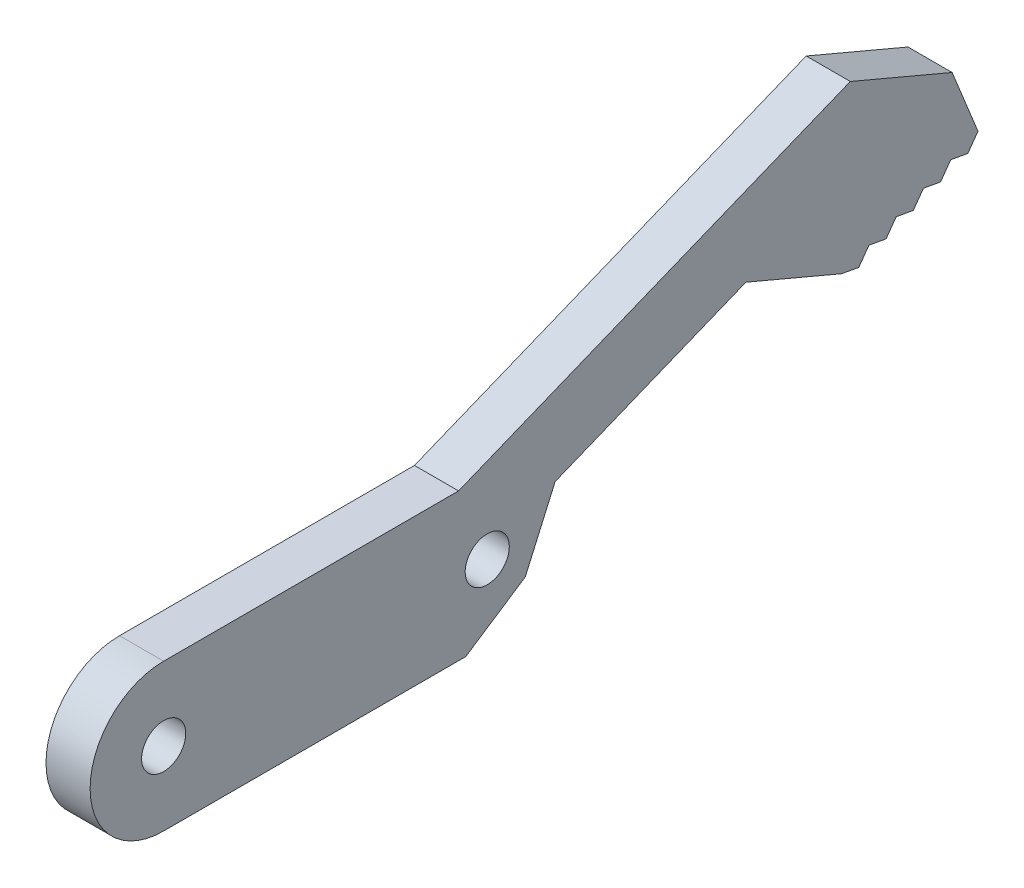
SolidWorks part; units mm, degrees
ref_plane "Front Plane" through (0, 0, 0) normal (0, 0, 1) x (1, 0, 0)
ref_plane "Top Plane" through (0, 0, 0) normal (0, 1, 0) x (1, 0, 0)
ref_plane "Right Plane" through (0, 0, 0) normal (1, 0, 0) x (0, 0, -1)
sketch "Sketch1" plane through (0, 0, 0) normal (1, 0, 0) x (0, 0, -1)
  line L1 (0, 0) -> (27, 0)
  line L2 (0, 0) -> (0, 10)
  line L3 (0, 10) -> (27, 10)
  circle A0 centre (5, 5) radius 1.5
  circle A1 centre (5, 5) radius 5
  circle A2 centre (27, 5) radius 5
  circle A3 centre (27, 5) radius 1.5
  dimension "D7" = 3
  dimension "D11" = 10
  dimension "D2" = 3
  dimension "D1" = 10
  dimension "D8" = 5
  dimension "D9" = 5
  dimension "D10" = 22
extrude "Boss-Extrude1" add sketch "Sketch1" along normal blind 3 contours A1 A0 | A2 L3 A1 L1 | A2 A3
sketch "Sketch2" plane through (3, 0, 0) normal (1, 0, 0) x (0, 0, -1)
  line L0 (27, 0) -> (60.3654, 13.5185)
  line L1 (5, 0) -> (27, 0) construction
  line L3 (60.3654, 13.5185) -> (56.6103, 22.7866)
  line L5 (56.6103, 22.7866) -> (25.0511, 10)
  line L6 (5, 10) -> (27, 10) construction
  line L7 (31.6102, 7.2627) -> (44.5856, 12.5199)
  line L8 (31.6102, 7.2627) -> (28.8536, 0.751)
  line L9 (44.5856, 12.5199) -> (51.0972, 9.7633)
  line L10 (51.0972, 9.7633) -> (60.3654, 13.5185)
  line L11 (51.0972, 9.7633) -> (51.3338, 9.1794)
  line L12 (60.3654, 13.5185) -> (60.602, 12.9346)
  line L13 (51.3338, 9.1794) -> (60.602, 12.9346)
  line L14 (5, 10) -> (27, 10)
  arc A3 (27, 0) -> (27, 10) centre (27, 5) ccw construction
  arc A4 (27, 0) -> (27, 10) centre (27, 5) ccw
  line M1 (27, 10) -> (5, 10)
  arc M4 (27, 0) -> (27, 10) centre (27, 5) ccw
  dimension "D1" = 157.944
  dimension "D2" = 36
  dimension "D3" = 90
  dimension "D4" = 10
  dimension "D5" = 10
  dimension "D6" = 45
  dimension "D7" = 45
  dimension "D8" = 5
  dimension "D9" = 5
  dimension "D10" = 14
  dimension "D11" = 0.63
extrude "Boss-Extrude2" add sketch "Sketch2" against normal blind 3 contours L7 L9 L0 L3 L5 L8 M1 M4 | L11 L13 L12 L0
sketch "Sketch4" plane through (3, 0, 0) normal (1, 0, 0) x (0, 0, -1)
  line L0 (51.6843, 20.7908) -> (58.6061, 17.8606)
  line L1 (56.6103, 22.7866) -> (25.0511, 10) construction
  line L2 (60.602, 12.9346) -> (56.6103, 22.7866) construction
  line L3 (44.5856, 12.5199) -> (51.0972, 9.7633) construction
  line L4 (56.6103, 22.7866) -> (25.0511, 10)
  line L5 (60.602, 12.9346) -> (56.6103, 22.7866)
  line M8 (60.602, 12.9346) -> (56.6103, 22.7866)
  line M9 (56.6103, 22.7866) -> (25.0511, 10)
extrude "Cut-Extrude2" cut sketch "Sketch4" against normal through all contours L0 M9 M8
sketch "Sketch5" plane through (3, 0, 0) normal (1, 0, 0) x (0, 0, -1)
  line L0 (31.5395, 7.0959) -> (29.5838, 2.665)
  line L1 (29.5838, 2.665) -> (25.5396, 0)
  line L2 (5, 0) -> (27, 0) construction
  line L3 (51.0972, 9.7633) -> (60.3654, 13.5185) construction
  line L4 (60.602, 12.9346) -> (58.6061, 17.8606) construction
  line L5 (51.0972, 9.7633) -> (52.2606, 9.5549)
  line L6 (51.3338, 9.1794) -> (60.602, 12.9346) construction
  line L7 (52.2606, 9.5549) -> (52.9509, 10.5144)
  line L8 (52.9509, 10.5144) -> (54.1143, 10.306)
  line L9 (54.1143, 10.306) -> (54.8045, 11.2654)
  line L10 (54.8045, 11.2654) -> (55.9679, 11.057)
  line L11 (55.9679, 11.057) -> (56.6582, 12.0164)
  line L12 (56.6582, 12.0164) -> (57.8215, 11.808)
  line L13 (57.8215, 11.808) -> (58.5118, 12.7674)
  line L14 (58.5118, 12.7674) -> (59.6752, 12.559)
  line L15 (59.6752, 12.559) -> (60.3654, 13.5185)
  line L16 (51.0972, 9.7633) -> (51.3338, 9.1794) construction
  line L17 (51.3338, 9.1794) -> (60.602, 12.9346)
  line L18 (51.0972, 9.7633) -> (51.3338, 9.1794)
  line L19 (60.602, 12.9346) -> (60.3654, 13.5185)
  line L20 (25.5396, 0) -> (27, 0)
  arc A0 (27, 0) -> (31.5395, 7.0959) centre (27, 5) ccw construction
  arc A1 (27, 0) -> (31.5395, 7.0959) centre (27, 5) ccw
  line M7 (5, 0) -> (27, 0)
  arc M8 (27, 0) -> (31.5395, 7.0959) centre (27, 5) ccw
  line M12 (51.0972, 9.7633) -> (51.3338, 9.1794)
  line M13 (51.3338, 9.1794) -> (60.602, 12.9346)
  line M14 (60.602, 12.9346) -> (58.6061, 17.8606)
  dimension "D1" = 4.8433
  dimension "D2" = 147.2
  dimension "D3" = 2
  dimension "D4" = 5
extrude "Cut-Extrude3" cut sketch "Sketch5" against normal blind 10 contours L0 L1 M7 M8 | L5 M12 M13 | L8 L7 M13 | L10 L9 M13 | L12 L11 M13 | L14 L13 M13 | L15 M13 M14
